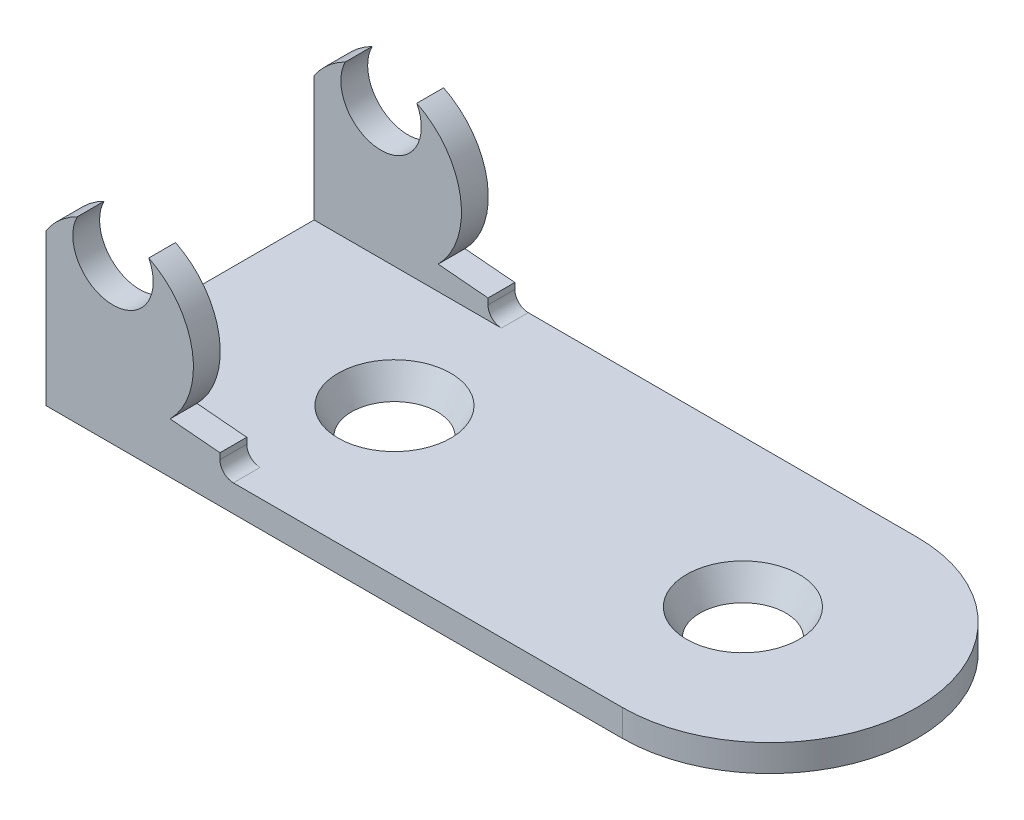
from build123d import *

# Parameters (mm, degrees)
BOSS_EXTRUDE1_DEPTH      = 5.5
BOSS_EXTRUDE1_DEPTH_BACK = 5.5
SKETCH2_W                = 108
SKETCH2_H                = 22
CUT_EXTRUDE1_DEPTH       = 11
SKETCH4_W                = 9
SKETCH4_H                = 10
CUT_EXTRUDE2_DEPTH       = 11


with BuildPart() as part:
    # Sketch1 → Boss-Extrude1 (new, two sides: drawn at the far end of the back side and taken through both)
    with BuildSketch(Plane.XY.offset(-BOSS_EXTRUDE1_DEPTH_BACK)):
        with BuildLine():
            Line((0, 0), (27, 0))
            Line((27, 0), (27, 1))
            Line((27, 1), (6.99, 1))
            ThreePointArc((6.99, 1), (6.636446609, 1.146446609), (6.49, 1.5))
            Line((6.49, 1.5), (6.49, 1.724666059))
            Line((6.49, 1.724666059), (4.63, 1.887394973))
            ThreePointArc((4.63, 1.887394973), (5.459499899, 4.491284383), (3.833170563, 6.6875))
            ThreePointArc((3.833170563, 6.6875), (2.5, 4.5), (1.166829437, 6.6875))
            ThreePointArc((1.166829437, 6.6875), (0.515533844, 6.249865346), (0, 5.658312395))
            Line((0, 5.658312395), (0, 0))
        make_face()
    extrude(amount=BOSS_EXTRUDE1_DEPTH + BOSS_EXTRUDE1_DEPTH_BACK)

    # Sketch2 → Cut-Extrude1 (cut)
    with BuildSketch(Plane(origin=(0, 0, 0), x_dir=(1, 0, 0), z_dir=(0, 1, 0))):
        Rectangle(SKETCH2_W, SKETCH2_H)
        with BuildLine():
            Line((0, 5.5), (0, -5.5))
            Line((0, -5.5), (21.5, -5.5))
            ThreePointArc((21.5, -5.5), (27, 0), (21.5, 5.5))
            Line((21.5, 5.5), (0, 5.5))
        make_face(mode=Mode.SUBTRACT)
    extrude(amount=CUT_EXTRUDE1_DEPTH, mode=Mode.SUBTRACT)

    # Sketch4 → Cut-Extrude2 (cut)
    with BuildSketch(Plane(origin=(0, 0, 0), x_dir=(0, 0, -1), z_dir=(1, 0, 0))):
        with Locations((0, 6)):
            Rectangle(SKETCH4_W, SKETCH4_H)
    extrude(amount=CUT_EXTRUDE2_DEPTH, mode=Mode.SUBTRACT)

    # Sketch3 → Cut-Revolve1 (revolve, cut)
    with BuildSketch(Plane.XY, mode=Mode.PRIVATE) as cut_revolve1_sk:
        Polygon((7.5, 1), (9.6, 1), (9.1, 0), (7.5, 0), align=None)
    revolve(cut_revolve1_sk.sketch.rotate(Axis((7.5, 0, 0), (0, 1, 0)), 270), axis=Axis((7.5, 0, 0), (0, 1, 0)), mode=Mode.SUBTRACT)

    # Sketch5 → Cut-Revolve2 (revolve, cut)
    with BuildSketch(Plane.XY, mode=Mode.PRIVATE) as cut_revolve2_sk:
        Polygon((20.5, 1), (22.6, 1), (22.1, 0), (20.5, 0), align=None)
    revolve(cut_revolve2_sk.sketch.rotate(Axis((20.5, 0, 0), (0, 1, 0)), 270), axis=Axis((20.5, 0, 0), (0, 1, 0)), mode=Mode.SUBTRACT)


solid = part.part
